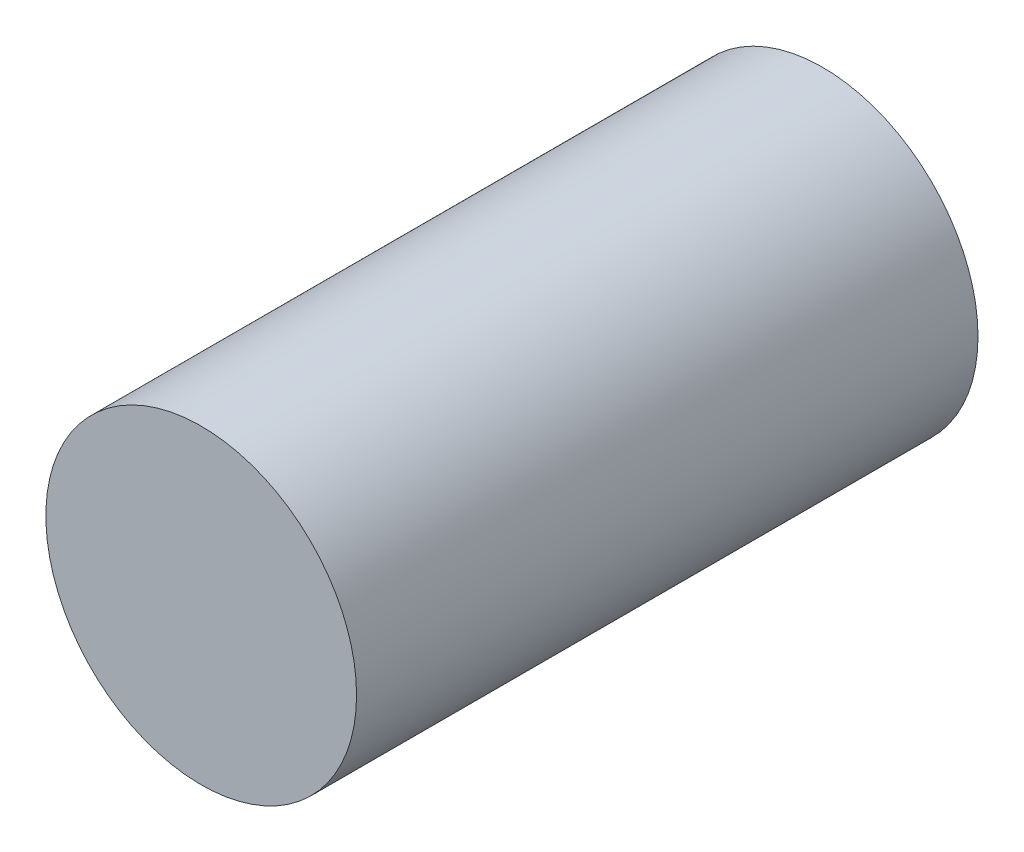
SolidWorks part; units mm, degrees
ref_plane "前视基准面" through (0, 0, 0) normal (0, 0, 1) x (1, 0, 0)
ref_plane "上视基准面" through (0, 0, 0) normal (0, 1, 0) x (1, 0, 0)
ref_plane "右视基准面" through (0, 0, 0) normal (1, 0, 0) x (0, 0, -1)
other "Configuration Table"
sketch "草图1" plane through (0, 0, 0) normal (0, 0, 1) x (1, 0, 0)
  circle A0 centre (0, 0) radius 8
  point P0 (0, 0)
  dimension "D1" = 16
extrude "凸台-拉伸1" add sketch "草图1" against normal mid plane 32
